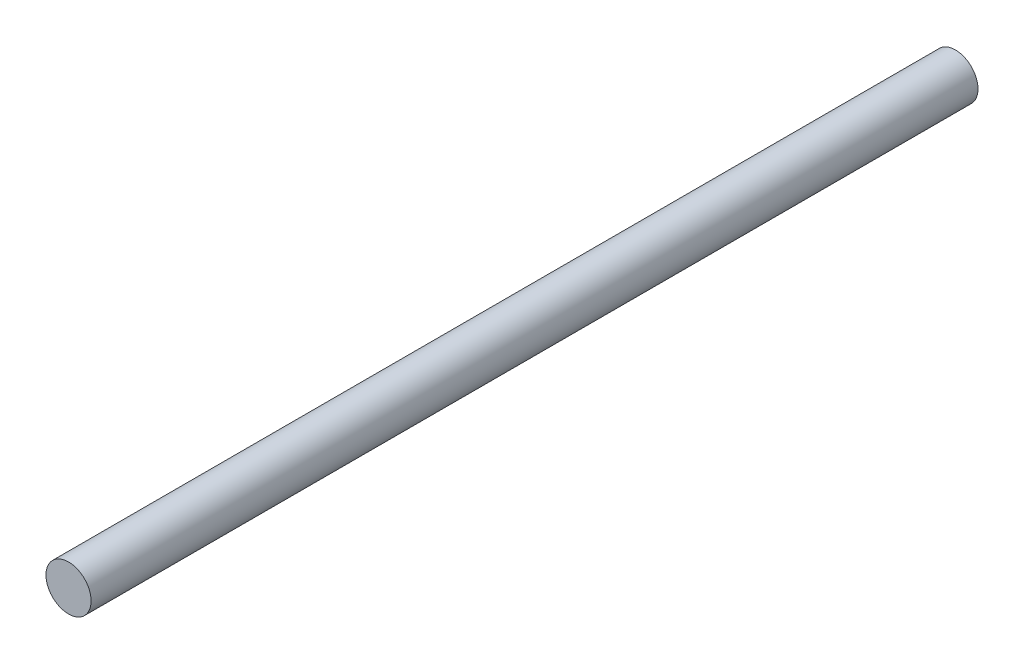
SolidWorks part; units mm, degrees
material "1.4000 (X6Cr13)"
ref_plane "Front Plane" through (0, 0, 0) normal (0, 0, 1) x (1, 0, 0)
ref_plane "Top Plane" through (0, 0, 0) normal (0, 1, 0) x (1, 0, 0)
ref_plane "Right Plane" through (0, 0, 0) normal (1, 0, 0) x (0, 0, -1)
sketch "Sketch1" plane through (0, 0, 0) normal (0, 0, 1) x (1, 0, 0)
  circle A0 centre (-151.119, -87.7318) radius 1.4
  dimension "D1" = 2.8
extrude "Boss-Extrude1" add sketch "Sketch1" along normal mid plane 55
